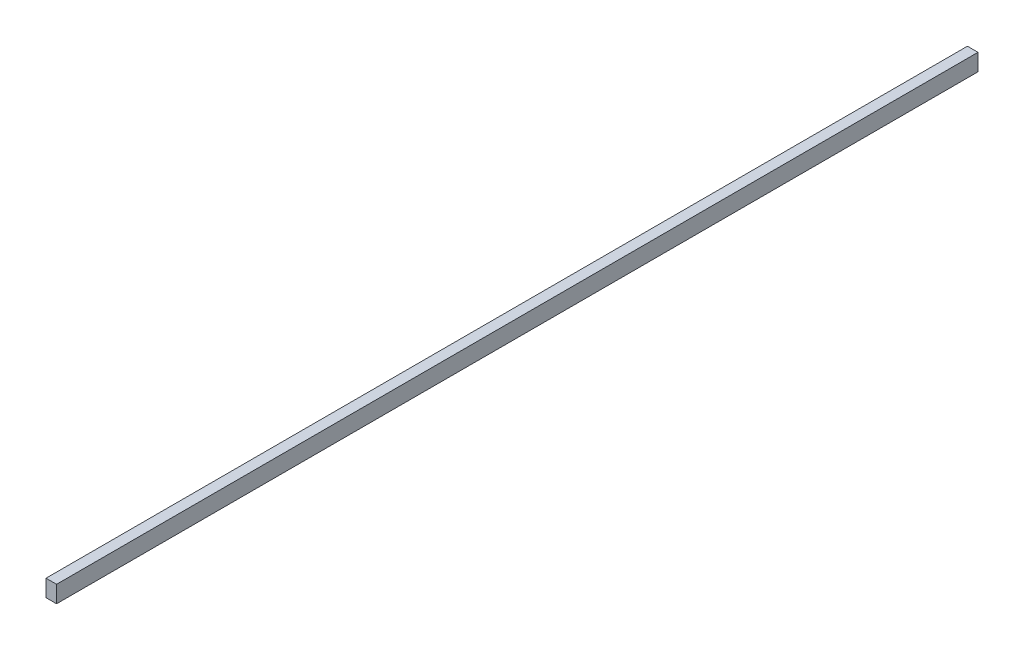
from build123d import *

# Parameters (mm, degrees)
SKETCH_1_W      = 25
SKETCH_1_H      = 40
EXTRUDE_1_DEPTH = 2180.980128516


with BuildPart() as part:
    # 草图1 → 凸台-拉伸1 (new body)
    with BuildSketch(Plane.XY):
        with Locations((-97.5, 0)):
            Rectangle(SKETCH_1_W, SKETCH_1_H)
    extrude(amount=EXTRUDE_1_DEPTH)


solid = part.part
